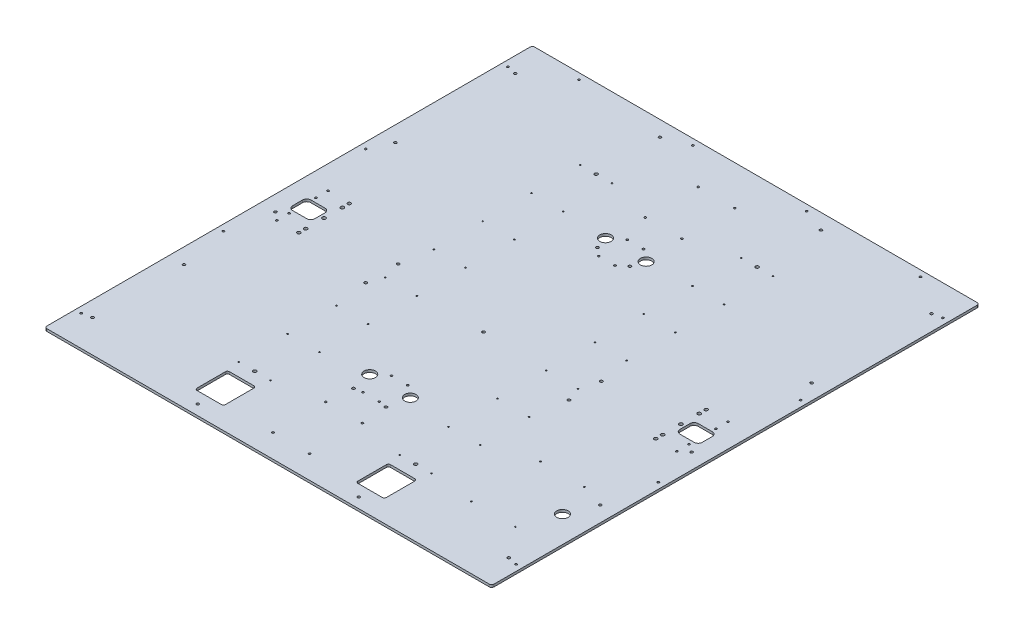
from build123d import *

# Parameters (mm, degrees)
SKETCH_1_W              = 1100
SKETCH_1_H              = 1200
EXTRUDE_1_DEPTH         = 6
FILLET_1_R              = 6
HOLE_WIZARD_M6_1_D      = 5
HOLE_WIZARD_8_0_8_1_D   = 8
HOLE_WIZARD_8_5_8_5_1_D = 8.5
CUT_EXTRUDE_1_DEPTH     = 10
HOLE_WIZARD_8_0_8_2_D   = 8
HOLE_WIZARD_M4_1_D      = 3.3
PATTERN_LINEAR_1_COUNT  = 8
PATTERN_LINEAR_1_PITCH  = 120
CUT_EXTRUDE_2_DEPTH     = 10
MIRROR_1_COPY_1_D       = 3.3
MIRROR_1_COPY_2_D       = 3.3
MIRROR_1_COPY_3_D       = 3.3
MIRROR_1_COPY_4_D       = 3.3
MIRROR_1_COPY_5_D       = 3.3
MIRROR_1_COPY_6_D       = 3.3
MIRROR_1_COPY_7_D       = 3.3
HOLE_WIZARD_M8_4_D      = 6.8
HOLE_WIZARD_6_5_6_5_1_D = 6.5
HOLE_WIZARD_6_5_6_5_2_D = 6.5
HOLE_WIZARD_M8_5_D      = 6.8
HOLE_WIZARD_6_5_6_5_3_D = 5
HOLE_WIZARD_M4_2_D      = 3.3
SKETCH_82_R             = 14
CUT_EXTRUDE_3_DEPTH     = 10
HOLE_WIZARD_M6_2_D      = 5
SKETCH_86_R             = 14
CUT_EXTRUDE_4_DEPTH     = 10


with BuildPart() as part:
    # 草图1 → 凸台-拉伸1 (new body)
    with BuildSketch(Plane(origin=(0, 0, 0), x_dir=(1, 0, 0), z_dir=(0, 1, 0))):
        Rectangle(SKETCH_1_W, SKETCH_1_H)
    extrude(amount=EXTRUDE_1_DEPTH)

    # 圆角1
    fillet_1_edges = [part.edges().sort_by_distance(p)[0] for p in [
        (550, 3, 600),
        (-550, 3, 600),
        (-550, 3, -600),
        (550, 3, -600),
    ]]
    fillet(fillet_1_edges, radius=FILLET_1_R)

    # M6 螺纹孔1 (through all)
    with Locations(Plane(origin=(0, 0, 0), x_dir=(-1, 0, 0), z_dir=(0, -1, 0))):
        with Locations((492, -86.500000001), (492, -56.500000001), (492, 9.499999999), (492, 39.499999999)):
            hole_wizard_m6_1 = Hole(HOLE_WIZARD_M6_1_D / 2)

    # Ø8.0 (8) 直径孔1 (through all)
    with Locations(Plane(origin=(0, 0, 0), x_dir=(-1, 0, 0), z_dir=(0, -1, 0))):
        with Locations((439, -85.500000001), (439, 38.499999999)):
            hole_wizard_8_0_8_1 = Hole(HOLE_WIZARD_8_0_8_1_D / 2)

    # Ø8.5 (8.5) 直径孔1 (through all)
    with Locations(Plane(origin=(0, 0, 0), x_dir=(-1, 0, 0), z_dir=(0, -1, 0))):
        with Locations((439, 21.499999999), (439, -23.500000001), (439, -68.500000001)):
            hole_wizard_8_5_8_5_1 = Hole(HOLE_WIZARD_8_5_8_5_1_D / 2)

    # 草图56 → 切除-拉伸1 (cut)
    with BuildSketch(Plane(origin=(0, 6, 0), x_dir=(1, 0, 0), z_dir=(0, 1, 0))):
        with BuildLine():
            Line((-494, -1.000000001), (-459, -1.000000001))
            ThreePointArc((-459, -1.000000001), (-451.928932188, -3.928932189), (-449, -11.000000001))
            Line((-449, -11.000000001), (-449, -36.000000001))
            ThreePointArc((-449, -36.000000001), (-451.928932188, -43.071067812), (-459, -46.000000001))
            Line((-459, -46.000000001), (-494, -46.000000001))
            ThreePointArc((-494, -46.000000001), (-501.071067812, -43.071067812), (-504, -36.000000001))
            Line((-504, -36.000000001), (-504, -11.000000001))
            ThreePointArc((-504, -11.000000001), (-501.071067812, -3.928932189), (-494, -1.000000001))
        make_face()
    cut_extrude_1 = extrude(amount=-CUT_EXTRUDE_1_DEPTH, mode=Mode.SUBTRACT)

    # Ø8.0 (8) 直径孔2 (through all)
    with Locations(Plane(origin=(0, 6, 0), x_dir=(1, 0, 0), z_dir=(0, 1, 0))):
        with Locations((-198, 405), (-198, -435)):
            hole_wizard_8_0_8_2 = Hole(HOLE_WIZARD_8_0_8_2_D / 2)

    # M4 螺纹孔1 (through all)
    with Locations(Plane(origin=(0, 6, 0), x_dir=(1, 0, 0), z_dir=(0, 1, 0))):
        with Locations((-159, -435), (-237, -435)):
            hole_wizard_m4_1 = Hole(HOLE_WIZARD_M4_1_D / 2)

    # 阵列(线性)1: M4 螺纹孔1 ×8
    with Locations(*[(0, 0, -i * PATTERN_LINEAR_1_PITCH) for i in range(1, PATTERN_LINEAR_1_COUNT)]):
        add(hole_wizard_m4_1, mode=Mode.SUBTRACT)

    # 草图59 → 切除-拉伸2 (cut)
    with BuildSketch(Plane(origin=(0, 6, 0), x_dir=(1, 0, 0), z_dir=(0, 1, 0))):
        with BuildLine():
            Line((-228, -467), (-168, -467))
            ThreePointArc((-168, -467), (-164.464466094, -468.464466094), (-163, -472))
            Line((-163, -472), (-163, -542))
            ThreePointArc((-163, -542), (-164.464466094, -545.535533906), (-168, -547))
            Line((-168, -547), (-228, -547))
            ThreePointArc((-228, -547), (-231.535533906, -545.535533906), (-233, -542))
            Line((-233, -542), (-233, -472))
            ThreePointArc((-233, -472), (-231.535533906, -468.464466094), (-228, -467))
        make_face()
    cut_extrude_2 = extrude(amount=-CUT_EXTRUDE_2_DEPTH, mode=Mode.SUBTRACT)

    # 镜向1: M6 螺纹孔1, Ø8.0 (8) 直径孔1, Ø8.5 (8.5) 直径孔1, 切除-拉伸1, Ø8.0 (8) 直径孔2, M4 螺纹孔1, 切除-拉伸2 across plane
    add(hole_wizard_m6_1.mirror(Plane(origin=(0, 0, 0), x_dir=(0, 0, 1), z_dir=(1, 0, 0))), mode=Mode.SUBTRACT)
    add(hole_wizard_8_0_8_1.mirror(Plane(origin=(0, 0, 0), x_dir=(0, 0, 1), z_dir=(1, 0, 0))), mode=Mode.SUBTRACT)
    add(hole_wizard_8_5_8_5_1.mirror(Plane(origin=(0, 0, 0), x_dir=(0, 0, 1), z_dir=(1, 0, 0))), mode=Mode.SUBTRACT)
    add(cut_extrude_1.mirror(Plane(origin=(0, 0, 0), x_dir=(0, 0, 1), z_dir=(1, 0, 0))), mode=Mode.SUBTRACT)
    add(hole_wizard_8_0_8_2.mirror(Plane(origin=(0, 0, 0), x_dir=(0, 0, 1), z_dir=(1, 0, 0))), mode=Mode.SUBTRACT)
    add(hole_wizard_m4_1.mirror(Plane(origin=(0, 0, 0), x_dir=(0, 0, 1), z_dir=(1, 0, 0))), mode=Mode.SUBTRACT)
    add(cut_extrude_2.mirror(Plane(origin=(0, 0, 0), x_dir=(0, 0, 1), z_dir=(1, 0, 0))), mode=Mode.SUBTRACT)

    # 镜向1 copy 1 (through all)
    with Locations(Plane(origin=(0, 6, -120), x_dir=(-1, 0, 0), z_dir=(0, 1, 0))):
        with Locations((-159, 435), (-237, 435)):
            Hole(MIRROR_1_COPY_1_D / 2)

    # 镜向1 copy 2 (through all)
    with Locations(Plane(origin=(0, 6, -240), x_dir=(-1, 0, 0), z_dir=(0, 1, 0))):
        with Locations((-159, 435), (-237, 435)):
            Hole(MIRROR_1_COPY_2_D / 2)

    # 镜向1 copy 3 (through all)
    with Locations(Plane(origin=(0, 6, -360), x_dir=(-1, 0, 0), z_dir=(0, 1, 0))):
        with Locations((-159, 435), (-237, 435)):
            Hole(MIRROR_1_COPY_3_D / 2)

    # 镜向1 copy 4 (through all)
    with Locations(Plane(origin=(0, 6, -480), x_dir=(-1, 0, 0), z_dir=(0, 1, 0))):
        with Locations((-159, 435), (-237, 435)):
            Hole(MIRROR_1_COPY_4_D / 2)

    # 镜向1 copy 5 (through all)
    with Locations(Plane(origin=(0, 6, -600), x_dir=(-1, 0, 0), z_dir=(0, 1, 0))):
        with Locations((-159, 435), (-237, 435)):
            Hole(MIRROR_1_COPY_5_D / 2)

    # 镜向1 copy 6 (through all)
    with Locations(Plane(origin=(0, 6, -720), x_dir=(-1, 0, 0), z_dir=(0, 1, 0))):
        with Locations((-159, 435), (-237, 435)):
            Hole(MIRROR_1_COPY_6_D / 2)

    # 镜向1 copy 7 (through all)
    with Locations(Plane(origin=(0, 6, -840), x_dir=(-1, 0, 0), z_dir=(0, 1, 0))):
        with Locations((-159, 435), (-237, 435)):
            Hole(MIRROR_1_COPY_7_D / 2)

    # M8 螺纹孔4 (through all)
    with Locations(Plane(origin=(0, 0, 0), x_dir=(-1, 0, 0), z_dir=(0, -1, 0))):
        with Locations((250, -30), (250, -110), (-250, -110), (-250, -30)):
            Hole(HOLE_WIZARD_M8_4_D / 2)

    # Ø6.5 (6.5) 直径孔1 (through all)
    with Locations(Plane(origin=(0, 6, 0), x_dir=(1, 0, 0), z_dir=(0, 1, 0))):
        with Locations((-512, -520), (-512, 520), (-512, -70), (-512, -295), (-512, 225)):
            hole_wizard_6_5_6_5_1 = Hole(HOLE_WIZARD_6_5_6_5_1_D / 2)

    # 镜向2: Ø6.5 (6.5) 直径孔1 across plane
    add(hole_wizard_6_5_6_5_1.mirror(Plane(origin=(0, 0, 0), x_dir=(0, 0, 1), z_dir=(1, 0, 0))), mode=Mode.SUBTRACT)

    # Ø6.5 (6.5) 直径孔2 (through all)
    with Locations(Plane(origin=(0, 6, 0), x_dir=(1, 0, 0), z_dir=(0, 1, 0))):
        with Locations((-198, -575), (0, -70), (-198, 562), (198, -575), (198, 562)):
            Hole(HOLE_WIZARD_6_5_6_5_2_D / 2)

    # M8 螺纹孔5 (through all)
    with Locations(Plane(origin=(0, 0, 0), x_dir=(-1, 0, 0), z_dir=(0, -1, 0))):
        with Locations((-40, 250), (40, 250), (-40, -350), (40, -350)):
            Hole(HOLE_WIZARD_M8_5_D / 2)

    # Ø6.5 (6.5) 直径孔3 (through all)
    with Locations(Plane(origin=(0, 6, 0), x_dir=(1, 0, 0), z_dir=(0, 1, 0))):
        with Locations((-535, 525), (-535, 175), (-535, -175), (-535, -525), (535, -525), (535, -175), (535, 175), (535, 525), (-140, 585), (140, 585), (-420, 585), (420, 585)):
            Hole(HOLE_WIZARD_6_5_6_5_3_D / 2)

    # M4 螺纹孔2 (through all)
    with Locations(Plane(origin=(0, 6, 0), x_dir=(1, 0, 0), z_dir=(0, 1, 0))):
        with Locations((454, -275.929836439), (454, -445.929836439), (346, -445.929836439), (346, -275.929836439)):
            Hole(HOLE_WIZARD_M4_2_D / 2)

    # 草图82 → 切除-拉伸3 (cut)
    with BuildSketch(Plane(origin=(0, 6, 0), x_dir=(1, 0, 0), z_dir=(0, 1, 0))):
        with Locations(Location((485, -360.929836439, 0), (0, 0, 270))):
            Circle(SKETCH_82_R)
    extrude(amount=-CUT_EXTRUDE_3_DEPTH, mode=Mode.SUBTRACT)

    # M6 螺纹孔2 (through all)
    with Locations(Plane(origin=(0, 6, 0), x_dir=(1, 0, 0), z_dir=(0, 1, 0))):
        with Locations((45, 373), (-45, -413), (-45, -543), (45, -413), (45, -543), (20, -276.5), (20, -346.5), (-20, -276.5), (-20, -346.5), (20, 303.5), (20, 233.5), (-20, 303.5), (-20, 233.5), (-45, 503), (-45, 373), (45, 503)):
            Hole(HOLE_WIZARD_M6_2_D / 2)

    # 草图86 → 切除-拉伸4 (cut)
    with BuildSketch(Plane(origin=(0, 6, 0), x_dir=(1, 0, 0), z_dir=(0, 1, 0))):
        with Locations(Location((50, 280, 0), (0, 0, 270))):
            Circle(SKETCH_86_R)
        with Locations(Location((-50, 280, 0), (0, 0, 270))):
            Circle(SKETCH_86_R)
        with Locations(Location((50, -300, 0), (0, 0, 270))):
            Circle(SKETCH_86_R)
        with Locations(Location((-50, -300, 0), (0, 0, 270))):
            Circle(SKETCH_86_R)
    extrude(amount=-CUT_EXTRUDE_4_DEPTH, mode=Mode.SUBTRACT)


solid = part.part
